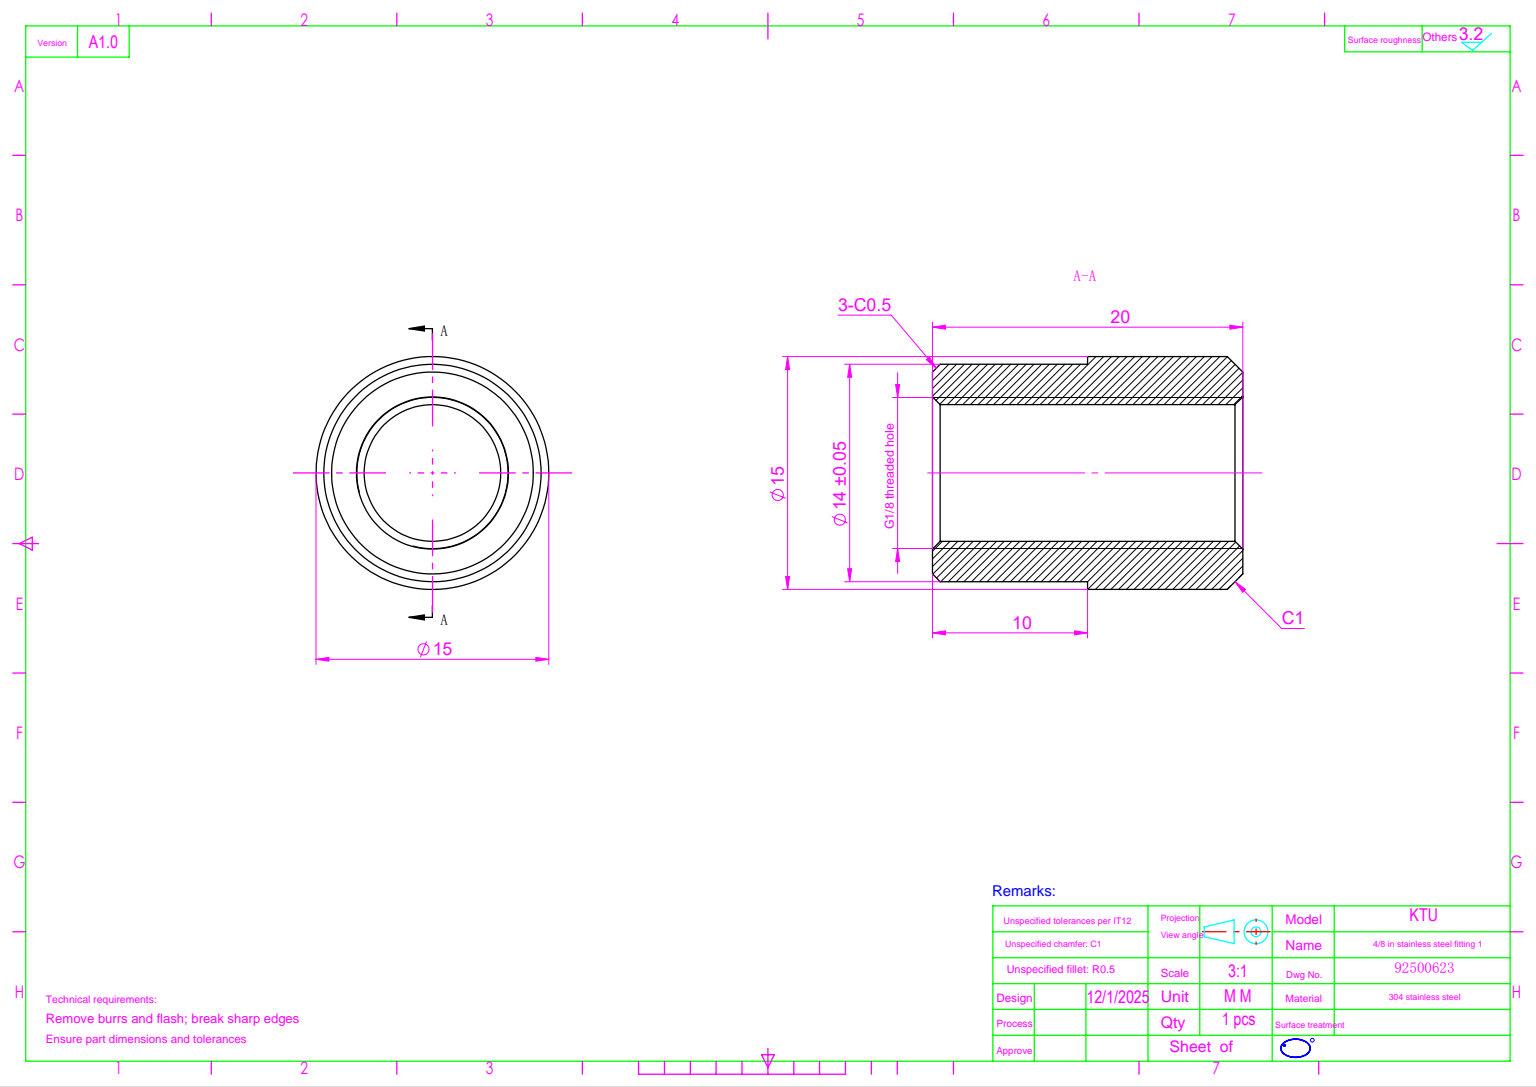
from build123d import *

# Parameters (mm, degrees)
SKETCH_1_R           = 7.5
EXTRUDE_1_DEPTH      = 20
SKETCH_2_OUTSIDE_W   = 22.83
SKETCH_2_OUTSIDE_H   = 22.83
SKETCH_2_OUTSIDE_R   = 7
CUT_EXTRUDE_1_DEPTH  = 10
HOLE_WIZARD_G1_8_1_D = 8.8
CHAMFER_1_SIZE       = 1
CHAMFER_2_SIZE       = 0.5


with BuildPart() as part:
    # 草图1 → 凸台-拉伸1 (new body)
    with BuildSketch(Plane.XY):
        Circle(SKETCH_1_R)
    extrude(amount=EXTRUDE_1_DEPTH)

    # 草图2 outside → 切除-拉伸1 (cut)
    with BuildSketch(Plane.XY.offset(20)):
        Rectangle(SKETCH_2_OUTSIDE_W, SKETCH_2_OUTSIDE_H)
        Circle(SKETCH_2_OUTSIDE_R, mode=Mode.SUBTRACT)
    extrude(amount=-CUT_EXTRUDE_1_DEPTH, mode=Mode.SUBTRACT)

    # G1/8 螺纹孔1 (through all)
    with Locations(Plane.XY.offset(20)):
        with Locations((0, 0)):
            Hole(HOLE_WIZARD_G1_8_1_D / 2)

    # 倒角1
    chamfer_1_edges = [part.edges().sort_by_distance(p)[0] for p in [
        (-7.5, 0, 0),
    ]]
    chamfer(chamfer_1_edges, length=CHAMFER_1_SIZE)

    # 倒角2
    chamfer_2_edges = [part.edges().sort_by_distance(p)[0] for p in [
        (-7, 0, 20),
        (4.4, 0, 20),
        (4.4, 0, 0),
    ]]
    chamfer(chamfer_2_edges, length=CHAMFER_2_SIZE)


solid = part.part
